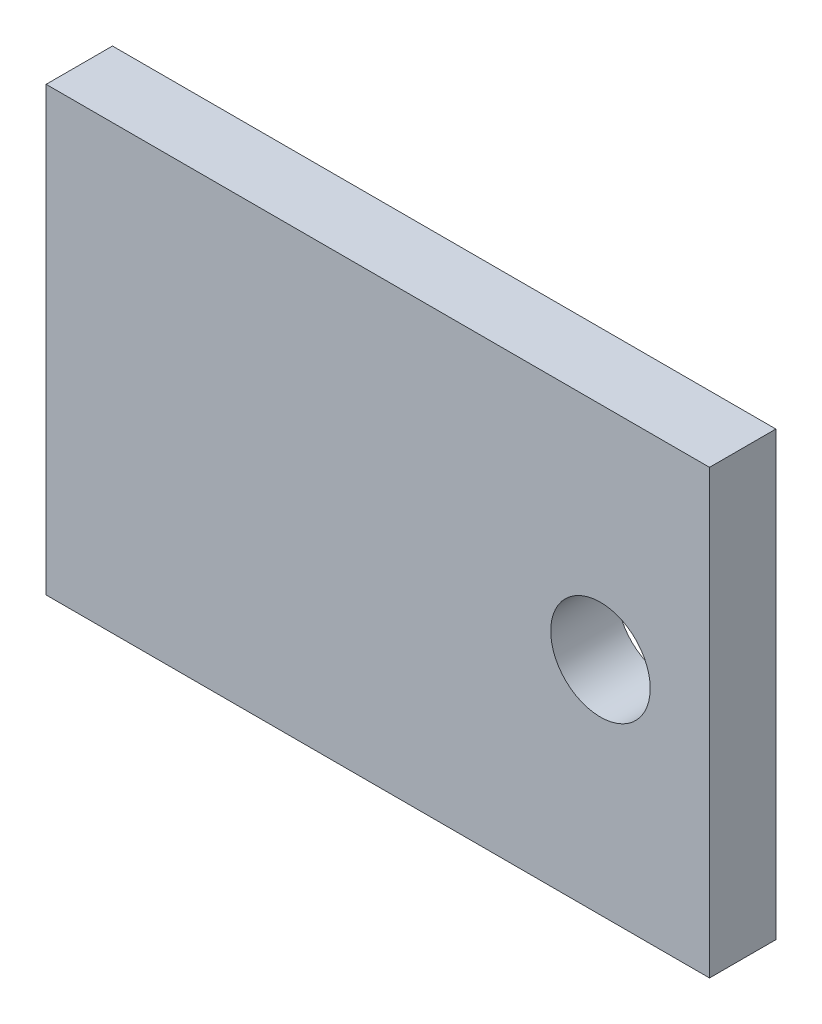
SolidWorks part; units mm, degrees
material "K"
ref_plane "Front" through (0, 0, 0) normal (0, 0, 1) x (1, 0, 0)
ref_plane "Top" through (0, 0, 0) normal (0, 1, 0) x (1, 0, 0)
ref_plane "Right" through (0, 0, 0) normal (1, 0, 0) x (0, 0, -1)
sketch "Sketch1" plane through (0, 0, 0) normal (0, 0, 1) x (1, 0, 0)
  line L1 (-30, -20) -> (30, -20)
  line L2 (-30, -20) -> (-30, 20)
  line L3 (-30, 20) -> (30, 20)
  line L4 (30, -20) -> (30, 20)
  line L5 (0, 20) -> (0, -20) construction
  line L6 (-30, 0) -> (30, 0) construction
  point P0 (0, 0)
  dimension "D1" = 60
  dimension "D2" = 40
extrude "Boss-Extrude1" add sketch "Sketch1" along normal blind 6
sketch "Sketch2" plane through (0, 0, 6) normal (0, 0, 1) x (1, 0, 0)
  circle A0 centre (20.1345, 0) radius 4.5
  dimension "D1" = 9
extrude "Cut-Extrude1" cut sketch "Sketch2" against normal blind 6
equation "\"零件重量\"= IIF ( \"SW-质量\" > 100 , int ( \"SW-质量\" ) , \"SW-质量\" )"
